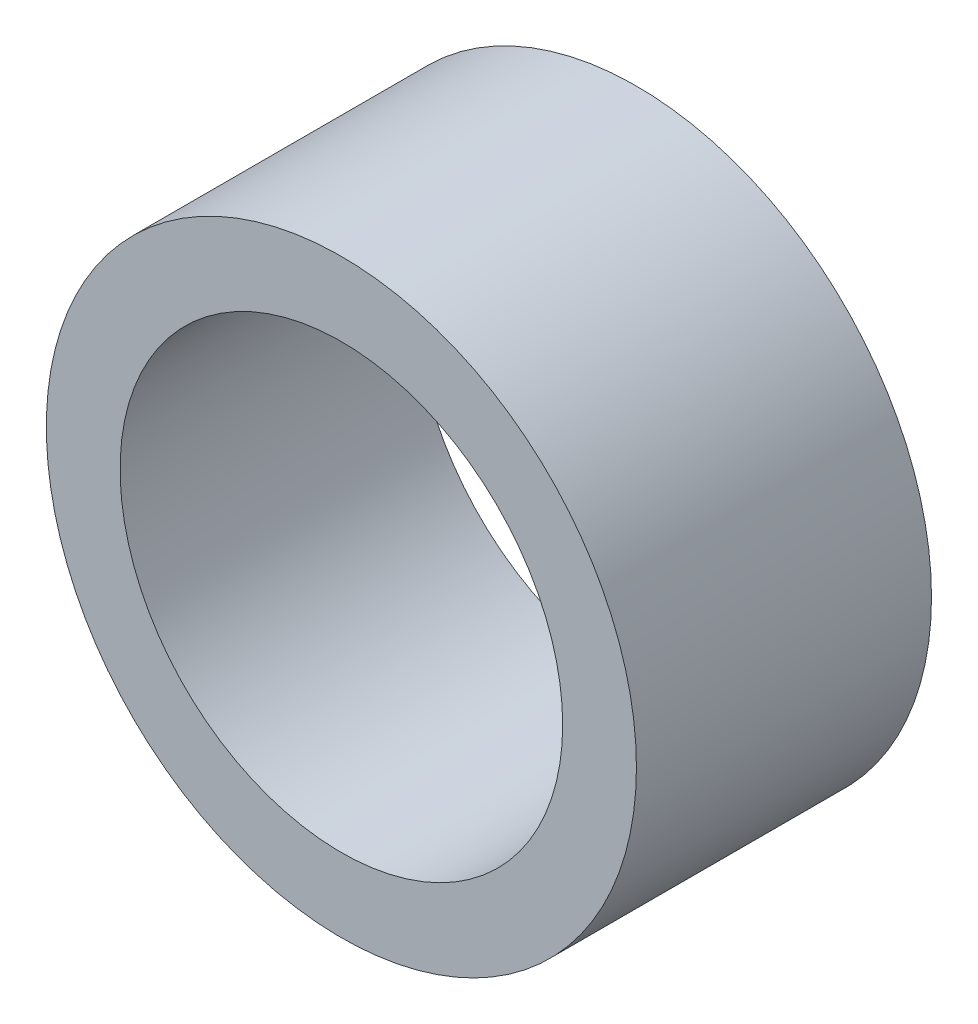
from build123d import *

# Parameters (mm, degrees)
SKETCH2_R           = 4
SKETCH2_R_2         = 3
BOSS_EXTRUDE1_DEPTH = 4


with BuildPart() as part:
    # Sketch2 → Boss-Extrude1 (new body)
    with BuildSketch(Plane.XY):
        Circle(SKETCH2_R)
        Circle(SKETCH2_R_2, mode=Mode.SUBTRACT)
    extrude(amount=BOSS_EXTRUDE1_DEPTH)


solid = part.part
